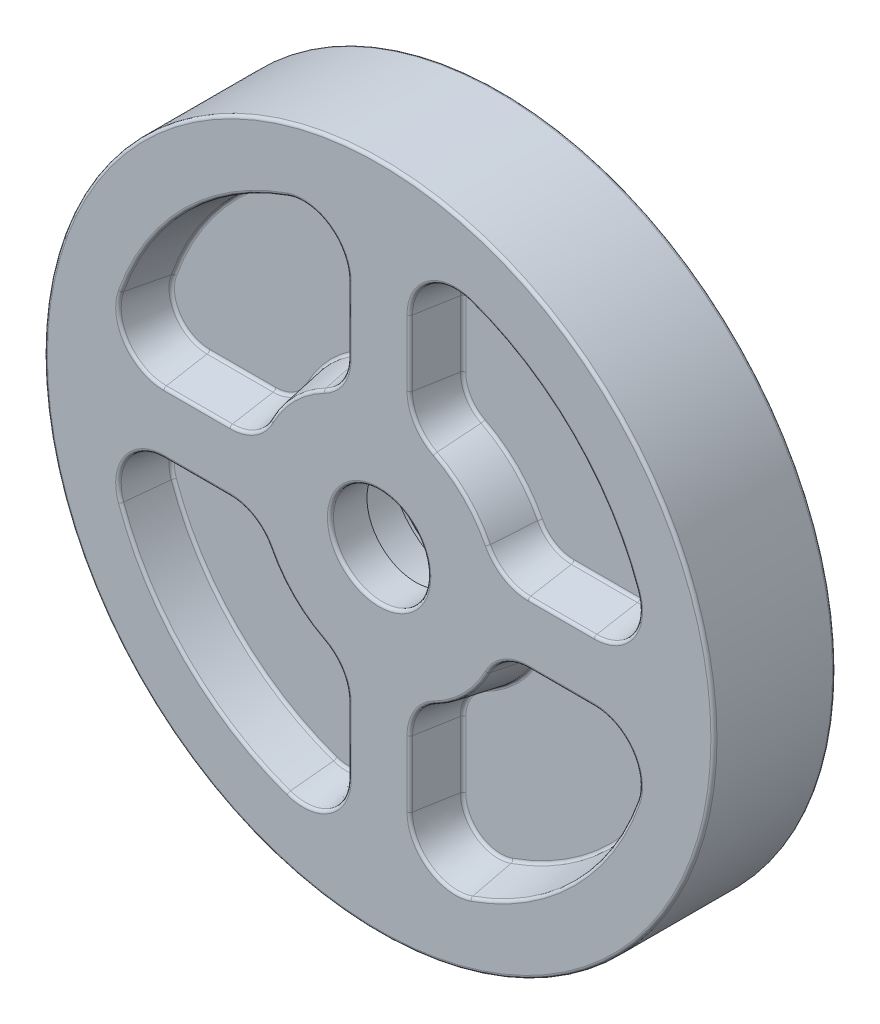
SolidWorks part; units mm, degrees
ref_plane "Front Plane" through (0, 0, 0) normal (0, 0, 1) x (1, 0, 0)
ref_plane "Top Plane" through (0, 0, 0) normal (0, 1, 0) x (1, 0, 0)
ref_plane "Right Plane" through (0, 0, 0) normal (1, 0, 0) x (0, 0, -1)
sketch "Sketch1" plane through (0, 0, 0) normal (0, 0, 1) x (1, 0, 0)
  circle A0 centre (0, 0) radius 110
  dimension "D1" = 220
extrude "Boss-Extrude1" add sketch "Sketch1" along normal mid plane 40
sketch "Sketch2" plane through (0, 0, 20) normal (0, 0, 1) x (1, 0, 0)
  circle A0 centre (0, 0) radius 16
  dimension "D1" = 32
extrude "Cut-Extrude1" cut sketch "Sketch2" against normal blind 12
sketch "Sketch3" plane through (0, 0, 8) normal (0, 0, 1) x (1, 0, 0)
  circle A0 centre (0, 0) radius 22.5
  dimension "D1" = 45
extrude "Cut-Extrude2" cut sketch "Sketch3" against normal blind 2
sketch "Sketch4" plane through (0, 0, 6) normal (0, 0, 1) x (1, 0, 0)
  circle A0 centre (0, 0) radius 26
  dimension "D1" = 52
extrude "Cut-Extrude3" cut sketch "Sketch4" against normal blind 15
sketch "Sketch5" plane through (0, 0, -9) normal (0, 0, 1) x (1, 0, 0)
  circle A0 centre (0, 0) radius 27.5
  dimension "D1" = 55
extrude "Cut-Extrude4" cut sketch "Sketch5" against normal blind 2
sketch "Sketch6" plane through (0, 0, -11) normal (0, 0, 1) x (1, 0, 0)
  circle A0 centre (0, 0) radius 26
  dimension "D1" = 52
extrude "Cut-Extrude5" cut sketch "Sketch6" against normal through all
sketch "Sketch7" plane through (0, 0, -20) normal (0, 0, -1) x (-1, 0, 0)
  line L1 (-10, 70.7107) -> (-10, 48.9898)
  line L7 (-70.7107, 10) -> (-48.9898, 10)
  arc A0 (-18.1818, 35.6289) -> (-35.6289, 18.1818) centre (0, 0) ccw
  arc A1 (-30, 84.8528) -> (-84.8528, 30) centre (0, 0) ccw
  arc A2 (-35.6289, 18.1818) -> (-48.9898, 10) centre (-48.9898, 25) cw
  arc A3 (-84.8528, 30) -> (-70.7107, 10) centre (-70.7107, 25) ccw
  arc A4 (-18.1818, 35.6289) -> (-10, 48.9898) centre (-25, 48.9898) ccw
  arc A5 (-10, 70.7107) -> (-30, 84.8528) centre (-25, 70.7107) ccw
  point P4 (0, 101.8147)
  point P5 (0, 31.4133)
  point P6 (-10, 101.8147)
  point P7 (-10, 31.4133)
  point P8 (10, 101.8147)
  point P9 (10, 31.4133)
  point P28 (0, 0)
  dimension "D1" = 80
  dimension "D2" = 180
  dimension "D3" = 15
extrude "Cut-Extrude6" cut sketch "Sketch7" against normal blind 15 draft 10
pattern_circular "CirPattern1" count 4 over 360 about axis through (0, 0, 0) along (0, 0, 1) of "Cut-Extrude6"
mirror "Mirror1" about plane through (0, 0, 0) normal (0, 0, 1) of "CirPattern1", "Cut-Extrude6"
fillet "Fillet1" radius 1 66 edges at (59.8502, 12.6449, -5) (80.7986, 17.8668, -5) (61.7694, 61.7694, -5) (17.8668, 80.7986, -5) (12.6449, 59.8502, -5) (14.4635, 42.5376, -5) (30.1545, 30.1545, -5) (42.5376, 14.4635, -5) (12.6449, -59.8502, -5) (17.8668, -80.7986, -5) (61.7694, -61.7694, -5) (80.7986, -17.8668, -5) (59.8502, -12.6449, -5) (42.5376, -14.4635, -5) (30.1545, -30.1545, -5) (14.4635, -42.5376, -5) (-59.8502, -12.6449, -5) (-80.7986, -17.8668, -5) (-61.7694, -61.7694, -5) (-17.8668, -80.7986, -5) (-12.6449, -59.8502, -5) (-14.4635, -42.5376, -5) (-30.1545, -30.1545, -5) (-42.5376, -14.4635, -5) (-12.6449, 59.8502, -5) (-17.8668, 80.7986, -5) (-61.7694, 61.7694, -5) (-80.7986, 17.8668, -5) (-59.8502, 12.6449, -5) (-42.5376, 14.4635, -5) (-30.1545, 30.1545, -5) (-14.4635, 42.5376, -5) (110, 0, -20) (26, 0, -20) (12.208, 41.1563, -20) (10, 59.8502, -20) (16.3397, 82.9581, -20) (63.6396, 63.6396, -20) (82.9581, 16.3397, -20) (59.8502, 10, -20) (41.1563, 12.208, -20) (28.2843, 28.2843, -20) (41.1563, -12.208, -20) (59.8502, -10, -20) (82.9581, -16.3397, -20) (63.6396, -63.6396, -20) (16.3397, -82.9581, -20) (10, -59.8502, -20) (12.208, -41.1563, -20) (28.2843, -28.2843, -20) (-12.208, -41.1563, -20) (-10, -59.8502, -20) (-16.3397, -82.9581, -20) (-63.6396, -63.6396, -20) (-82.9581, -16.3397, -20) (-59.8502, -10, -20) (-41.1563, -12.208, -20) (-28.2843, -28.2843, -20) (-41.1563, 12.208, -20) (-59.8502, 10, -20) (-82.9581, 16.3397, -20) (-63.6396, 63.6396, -20) (-16.3397, 82.9581, -20) (-10, 59.8502, -20) (-12.208, 41.1563, -20) (-28.2843, 28.2843, -20)
fillet "Fillet2" radius 1 66 edges at (-30.1545, -30.1545, 5) (-14.4635, -42.5376, 5) (-12.6449, -59.8502, 5) (-17.8668, -80.7986, 5) (-61.7694, -61.7694, 5) (-80.7986, -17.8668, 5) (-59.8502, -12.6449, 5) (-42.5376, -14.4635, 5) (30.1545, -30.1545, 5) (42.5376, -14.4635, 5) (59.8502, -12.6449, 5) (80.7986, -17.8668, 5) (61.7694, -61.7694, 5) (17.8668, -80.7986, 5) (12.6449, -59.8502, 5) (14.4635, -42.5376, 5) (30.1545, 30.1545, 5) (14.4635, 42.5376, 5) (12.6449, 59.8502, 5) (17.8668, 80.7986, 5) (61.7694, 61.7694, 5) (80.7986, 17.8668, 5) (59.8502, 12.6449, 5) (42.5376, 14.4635, 5) (-30.1545, 30.1545, 5) (-42.5376, 14.4635, 5) (-59.8502, 12.6449, 5) (-80.7986, 17.8668, 5) (-61.7694, 61.7694, 5) (-17.8668, 80.7986, 5) (-12.6449, 59.8502, 5) (-14.4635, 42.5376, 5) (-16.3397, 82.9581, 20) (-63.6396, 63.6396, 20) (-82.9581, 16.3397, 20) (-59.8502, 10, 20) (-41.1563, 12.208, 20) (-28.2843, 28.2843, 20) (-12.208, 41.1563, 20) (-10, 59.8502, 20) (16.3397, -82.9581, 20) (63.6396, -63.6396, 20) (82.9581, -16.3397, 20) (59.8502, -10, 20) (41.1563, -12.208, 20) (28.2843, -28.2843, 20) (12.208, -41.1563, 20) (10, -59.8502, 20) (110, 0, 20) (16, 0, 20) (82.9581, 16.3397, 20) (63.6396, 63.6396, 20) (16.3397, 82.9581, 20) (10, 59.8502, 20) (12.208, 41.1563, 20) (28.2843, 28.2843, 20) (41.1563, 12.208, 20) (59.8502, 10, 20) (-82.9581, -16.3397, 20) (-63.6396, -63.6396, 20) (-16.3397, -82.9581, 20) (-10, -59.8502, 20) (-12.208, -41.1563, 20) (-28.2843, -28.2843, 20) (-41.1563, -12.208, 20) (-59.8502, -10, 20)
sketch "Sketch8" plane through (0, 0, -20) normal (0, 0, -1) x (-1, 0, 0)
  circle A1 centre (0, 32.5) radius 1.5
  circle A2 centre (28.1458, -16.25) radius 1.5
  circle A3 centre (-28.1458, -16.25) radius 1.5
  point P11 (0, 0)
  dimension "D2" = 3
  dimension "D3" = 3
extrude "Cut-Extrude7" cut sketch "Sketch8" against normal blind 10
